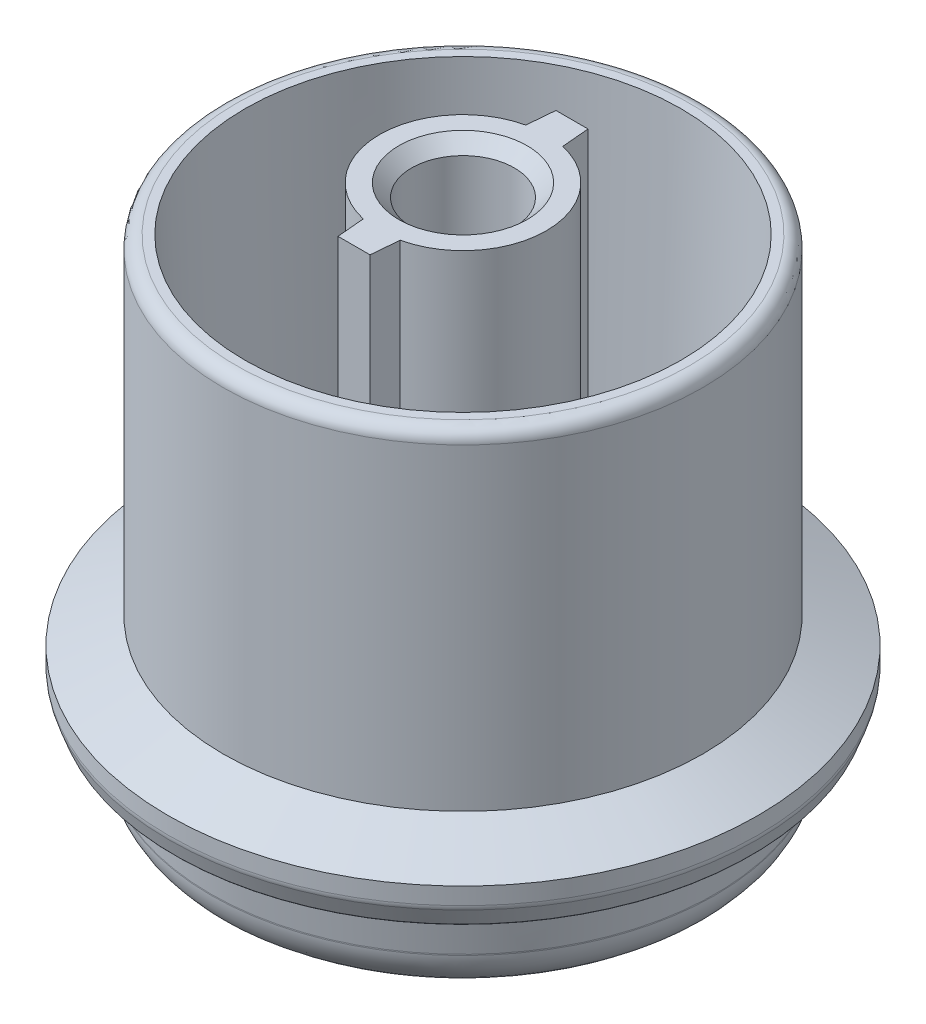
SolidWorks part; units mm, degrees
material "H62黄铜"
ref_plane "Front Plane" through (0, 0, 0) normal (0, 0, 1) x (1, 0, 0)
ref_plane "Top Plane" through (0, 0, 0) normal (0, 1, 0) x (1, 0, 0)
ref_plane "Right Plane" through (0, 0, 0) normal (1, 0, 0) x (0, 0, -1)
sketch "Sketch2" plane through (0, 0, 0) normal (0, 0, 1) x (1, 0, 0)
  line L0 (0, 76) -> (0, -54.3322) construction
  line L1 (0, 0) -> (40, 0)
  line L2 (40, 0) -> (40, 14.5)
  line L3 (40, 14.5) -> (46, 14.5)
  line L4 (46, 14.5) -> (46, 20.5)
  line L5 (46, 20.5) -> (37.4, 24.5102)
  line L6 (37.4, 24.5102) -> (37.4, 76)
  line L7 (37.4, 76) -> (0, 76)
  line L8 (0, 76) -> (0, 0)
  dimension "D1" = 40
  dimension "D2" = 14.5
  dimension "D3" = 46
  dimension "D4" = 20.5
  dimension "D5" = 25
  dimension "D6" = 37.4
  dimension "D7" = 76
revolve "Revolve1" add sketch "Sketch2" angle 360 about L0
chamfer "Chamfer1" distance 3 angle 20 1 edges at (-46, 14.5, 0)
sketch "Sketch3" plane through (0, 0, 0) normal (0, 0, 1) x (1, 0, 0)
  line L0 (0, 134.9167) -> (0, -55.0936) construction
  line L1 (34, 76) -> (0, 76)
  line L2 (37.4, 76) -> (-37.4, 76) construction
  line L3 (34, 76) -> (31.6254, 8)
  line L4 (31.6254, 8) -> (0, 8)
  line L5 (0, 8) -> (0, 76)
  dimension "D1" = 68
  dimension "D2" = 2
  dimension "D3" = 34
revolve "Cut-Revolve1" cut sketch "Sketch3" angle 360 about L0
sketch "Sketch4" plane through (0, 8, 0) normal (0, 1, 0) x (1, 0, 0)
  circle A0 centre (0, 0) radius 13
  dimension "D1" = 26
extrude "Boss-Extrude1" add sketch "Sketch4" along normal blind 75
sketch "Sketch5" plane through (0, 8, 0) normal (0, 1, 0) x (1, 0, 0)
  line L0 (0, 78.6067) -> (0, -76.4641) construction
  line L1 (-72.7145, 0) -> (86.9092, 0) construction
  line L2 (-2.5, 17) -> (-2.8782, 12.6774)
  line L3 (-2.5, 17) -> (2.5, 17)
  line L4 (2.5, 17) -> (2.8782, 12.6774)
  arc A2 (2.8782, 12.6774) -> (-2.8782, 12.6774) centre (0, 0) ccw
  circle A3 centre (0, 0) radius 13 construction
  dimension "D1" = 5
  dimension "D2" = 5
  dimension "D3" = 17
extrude "Boss-Extrude2" add sketch "Sketch5" along normal up to surface (75 mm away) up to face at (0, 83, 13)
pattern_circular "CirPattern1" count 2 over 360 about axis through (0, 0, 0) along (0, 1, 0) of "Boss-Extrude2"
fillet "Fillet1" radius 2 1 edges at (0, 8, 31.6254)
fillet "Fillet2" radius 2 1 edges at (-37.4, 76, 0)
sketch "Sketch6" plane through (0, 0, 0) normal (1, 0, 0) x (0, 0, -1)
  line L0 (0, 140.4888) -> (0, -85.672) construction
  line L1 (12.6774, 83) -> (-12.6774, 83) construction
  line L2 (0, 58) -> (10, 58)
  line L3 (0, 58) -> (0, 26)
  line L4 (0, 26) -> (10, 26)
  line L5 (10, 58) -> (10, 26)
  dimension "D1" = 10
  dimension "D2" = 25
  dimension "D3" = 57
revolve "Cut-Revolve2" cut sketch "Sketch6" angle 360 about L0
sketch "Sketch7" plane through (0, 83, 0) normal (0, 1, 0) x (1, 0, 0)
  circle A0 centre (0, 0) radius 8
  dimension "D1" = 16
extrude "Cut-Extrude1" cut sketch "Sketch7" against normal blind 30
sketch "Sketch8" plane through (0, 0, 0) normal (0, -1, 0) x (1, 0, 0)
  line L0 (-74.2099, 0) -> (72.2012, 0) construction
  line L1 (0, 58.8099) -> (0, -68.8534) construction
  circle A0 centre (-20, 0) radius 3
  circle A1 centre (20, 0) radius 3
  dimension "D1" = 6
  dimension "D2" = 40
extrude "Cut-Extrude2" cut sketch "Sketch8" against normal blind 30
chamfer "Chamfer2" distance 2 angle 45 1 edges at (0, 83, 8)
sketch "Sketch9" plane through (0, 0, 0) normal (0, -1, 0) x (1, 0, 0)
  circle A0 centre (0, 0) radius 10
  dimension "D1" = 20
extrude "Cut-Extrude3" cut sketch "Sketch9" against normal blind 10
chamfer "Chamfer3" distance 1 angle 45 1 edges at (10, 0, 0)
sketch "Sketch10" plane through (0, 0, 0) normal (0, 0, 1) x (1, 0, 0)
  line L0 (0, 143.9682) -> (0, -73.842) construction
  line L1 (-43.4, 14.5) -> (-43.4, 18)
  line L2 (-44.9081, 14.5) -> (44.9081, 14.5) construction
  line L3 (-43.4, 18) -> (-40.65, 18)
  line L4 (-39.4426, 16.4265) -> (-39.7838, 15.1532)
  line L6 (-40, 14.5) -> (-40, 0) construction
  line L7 (-43.4, 14.5) -> (-43.4, 0)
  line L8 (-40, 13.6) -> (-39.335, 6.57)
  line L9 (-39.335, 6.57) -> (-38.7602, 0)
  line L11 (-38.7602, 0) -> (-43.4, 0)
  arc A0 (-40.65, 18) -> (-39.4426, 16.4265) centre (-40.65, 16.75) cw
  arc A1 (-39.7838, 15.1532) -> (-39.6816, 14.9234) centre (-39.5906, 15.1015) ccw
  arc A2 (-39.6816, 14.9234) -> (-40, 13.6) centre (-40, 14.3) cw
  dimension "D3" = 1.25
  dimension "D6" = 0.2
  dimension "D7" = 3.7
  dimension "D8" = 0.7
  dimension "D9" = 4.1
  dimension "D10" = 39.335
  dimension "D1" = 43.4
  dimension "D2" = 3.5
  dimension "D4" = 15
  dimension "D5" = 4
  dimension "D11" = 7.03
  dimension "D12" = 5
revolve "Cut-Revolve3" cut sketch "Sketch10" angle 360 about L0
fillet "Fillet3" radius 7 1 edges at (0, 0, 38.7602)
fillet "Fillet4" radius 2 1 edges at (-46, 17.5, 0)
fillet "Fillet5" radius 0.2 2 edges at (-43.4, 14.5, 0) (-44.9081, 14.5, 0)
fillet "Fillet6" radius 1.25 1 edges at (0, 18, 43.4)
fillet "Fillet7" radius 0.2 1 edges at (0, 13.6, 40)
